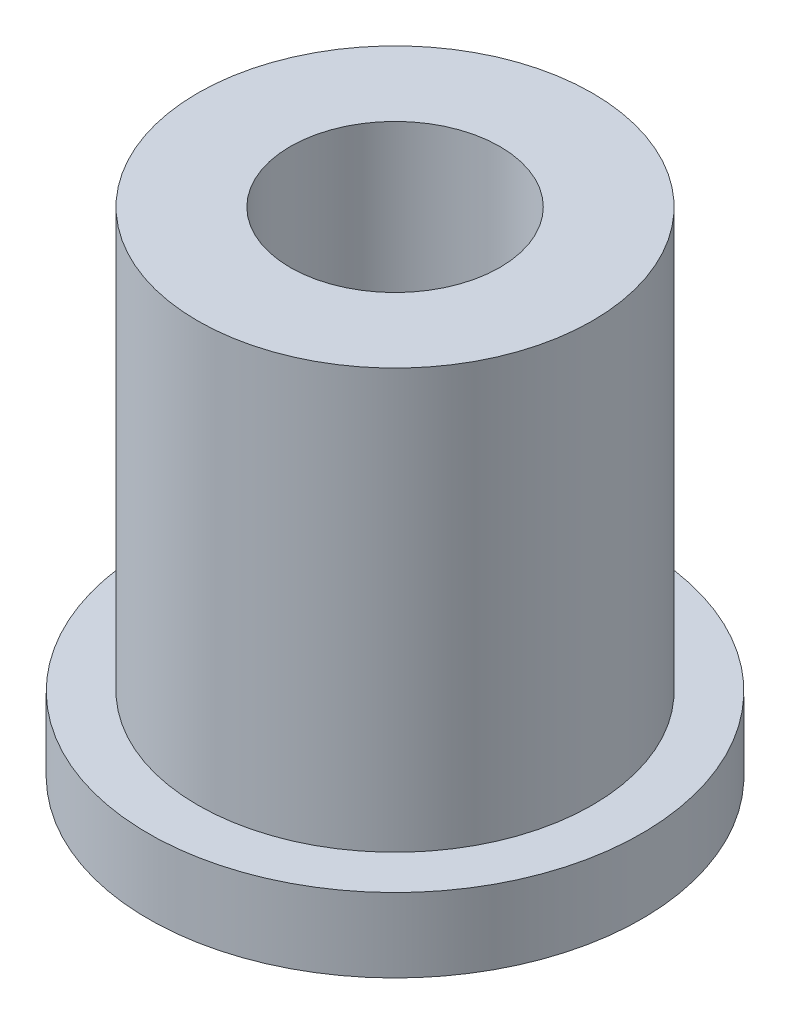
SolidWorks part; units mm, degrees
material "Q235"
ref_plane "Front Plane" through (0, 0, 0) normal (0, 0, 1) x (1, 0, 0)
ref_plane "Top Plane" through (0, 0, 0) normal (0, 1, 0) x (1, 0, 0)
ref_plane "Right Plane" through (0, 0, 0) normal (1, 0, 0) x (0, 0, -1)
sketch "Sketch1" plane through (0, 0, 0) normal (0, 1, 0) x (1, 0, 0)
  circle A0 centre (0, 0) radius 8
  dimension "D1" = 16
extrude "Boss-Extrude1" add sketch "Sketch1" along normal blind 20
hole_wizard "M10 Tapped Hole1" positions "Sketch3" profile "Sketch2" tap size "M10" standard "Gb"
sketch "Sketch3" plane through (0, 20, 0) normal (0, 1, 0) x (1, 0, 0)
  point P0 (0, 0)
sketch "Sketch2" plane through (0, 20, 0) normal (1, 0, 0) x (0, 0, 1)
  line L0 (0, 0) -> (0, 27.0537)
  line L1 (0, 27.0537) -> (4.25, 24.5)
  line L2 (4.25, 24.5) -> (4.25, 0)
  line L5 (4.25, 0) -> (0, 0)
  line L10 (0, 27.0537) -> (-4.25, 24.5) construction
  line L11 (0, -6.35) -> (0, 107.95) construction
  dimension "螺纹孔钻头直径" = 8.5
  dimension "螺纹孔钻头深度" = 24.5
  dimension "导头角度" = 118
cosmetic thread "Cosmetic Thread1" parameters "D1"=20, "D2"=10
sketch "Sketch4" plane through (0, 0, 0) normal (0, -1, 0) x (1, 0, 0)
  circle A0 centre (0, 0) radius 10
  circle A1 centre (0, 0) radius 8
  dimension "D1" = 20
extrude "Boss-Extrude3" add sketch "Sketch4" against normal blind 3
